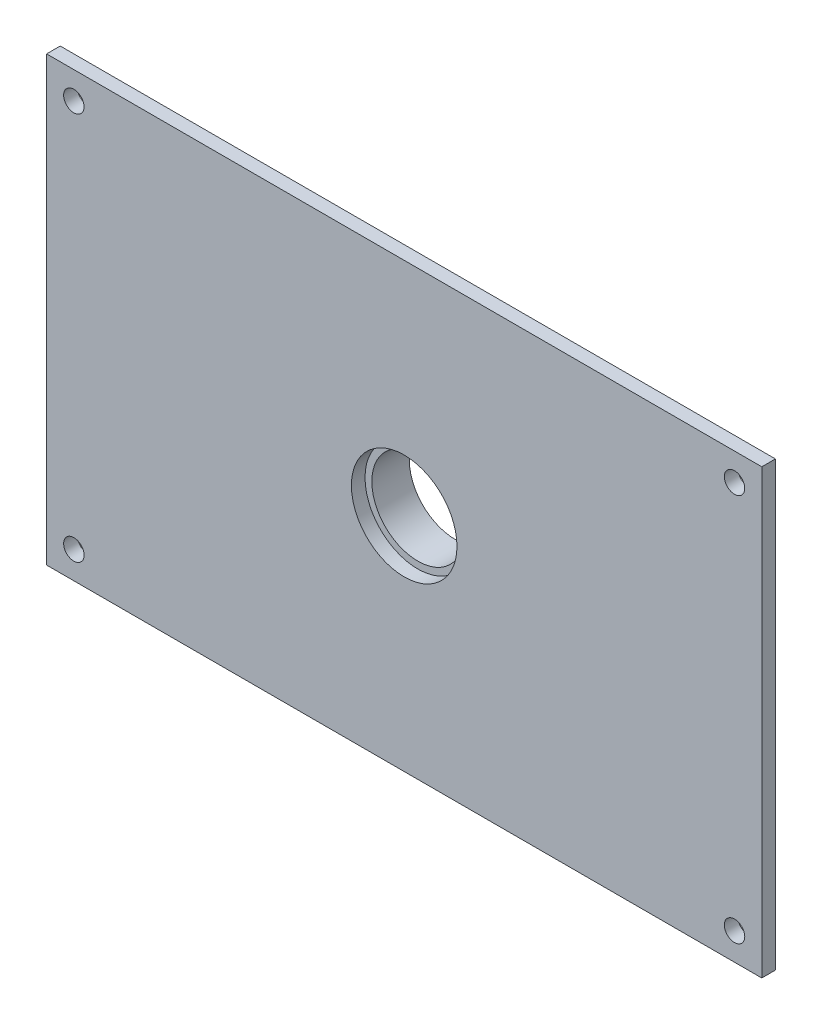
SolidWorks part; units mm, degrees
ref_plane "Front" through (0, 0, 0) normal (0, 0, 1) x (1, 0, 0)
ref_plane "Top" through (0, 0, 0) normal (0, 1, 0) x (1, 0, 0)
ref_plane "Right" through (0, 0, 0) normal (1, 0, 0) x (0, 0, -1)
sketch "Sketch1" plane through (0, 0, 0) normal (0, 0, 1) x (1, 0, 0)
  line L0 (-97, 88.9691) -> (-97, -98.4517) construction
  line L1 (-105, 65) -> (105, 65)
  line L2 (-105, 65) -> (-105, -65)
  line L3 (-105, -65) -> (105, -65)
  line L4 (105, 65) -> (105, -65)
  line L5 (97, 109.2308) -> (97, -98.4517) construction
  line L6 (131.1437, 57) -> (-128.5746, 57) construction
  line L7 (134.3672, -57) -> (-143.3104, -57) construction
  circle A0 centre (97, 57) radius 3
  circle A1 centre (-97, 57) radius 3
  circle A2 centre (-97, -57) radius 3
  circle A3 centre (97, -57) radius 3
  dimension "D9" = 6
  dimension "D10" = 6
  dimension "D11" = 6
  dimension "D12" = 6
  dimension "D1" = 130
  dimension "D2" = 210
  dimension "D3" = 65
  dimension "D4" = 105
  dimension "D5" = 8
  dimension "D6" = 8
  dimension "D7" = 8
  dimension "D8" = 8
extrude "Boss-Extrude1" add sketch "Sketch1" along normal blind 4
sketch "Sketch2" plane through (0, 0, 0) normal (0, 0, -1) x (-1, 0, 0)
  line L1 (-24, 24) -> (24, 24)
  line L2 (-24, 24) -> (-24, -24)
  line L3 (-24, -24) -> (24, -24)
  line L4 (24, 24) -> (24, -24)
  dimension "D1" = 48
  dimension "D2" = 24
  dimension "D3" = 48
  dimension "D4" = 24
extrude "Boss-Extrude2" add sketch "Sketch2" along normal blind 11
sketch "Sketch3" plane through (0, 0, -11) normal (0, 0, -1) x (-1, 0, 0)
  circle A0 centre (0, 0) radius 13.5
  dimension "D1" = 27
extrude "Cut-Extrude1" cut sketch "Sketch3" against normal blind 11
sketch "Sketch4" plane through (0, 0, 0) normal (0, 0, -1) x (-1, 0, 0)
  circle A0 centre (0, 0) radius 15.5
  dimension "D1" = 31
extrude "Cut-Extrude2" cut sketch "Sketch4" against normal blind 11
scale "Scale 1" bodies to scale 104 scale about centroid uniform scaling yes scale factor 1.875
